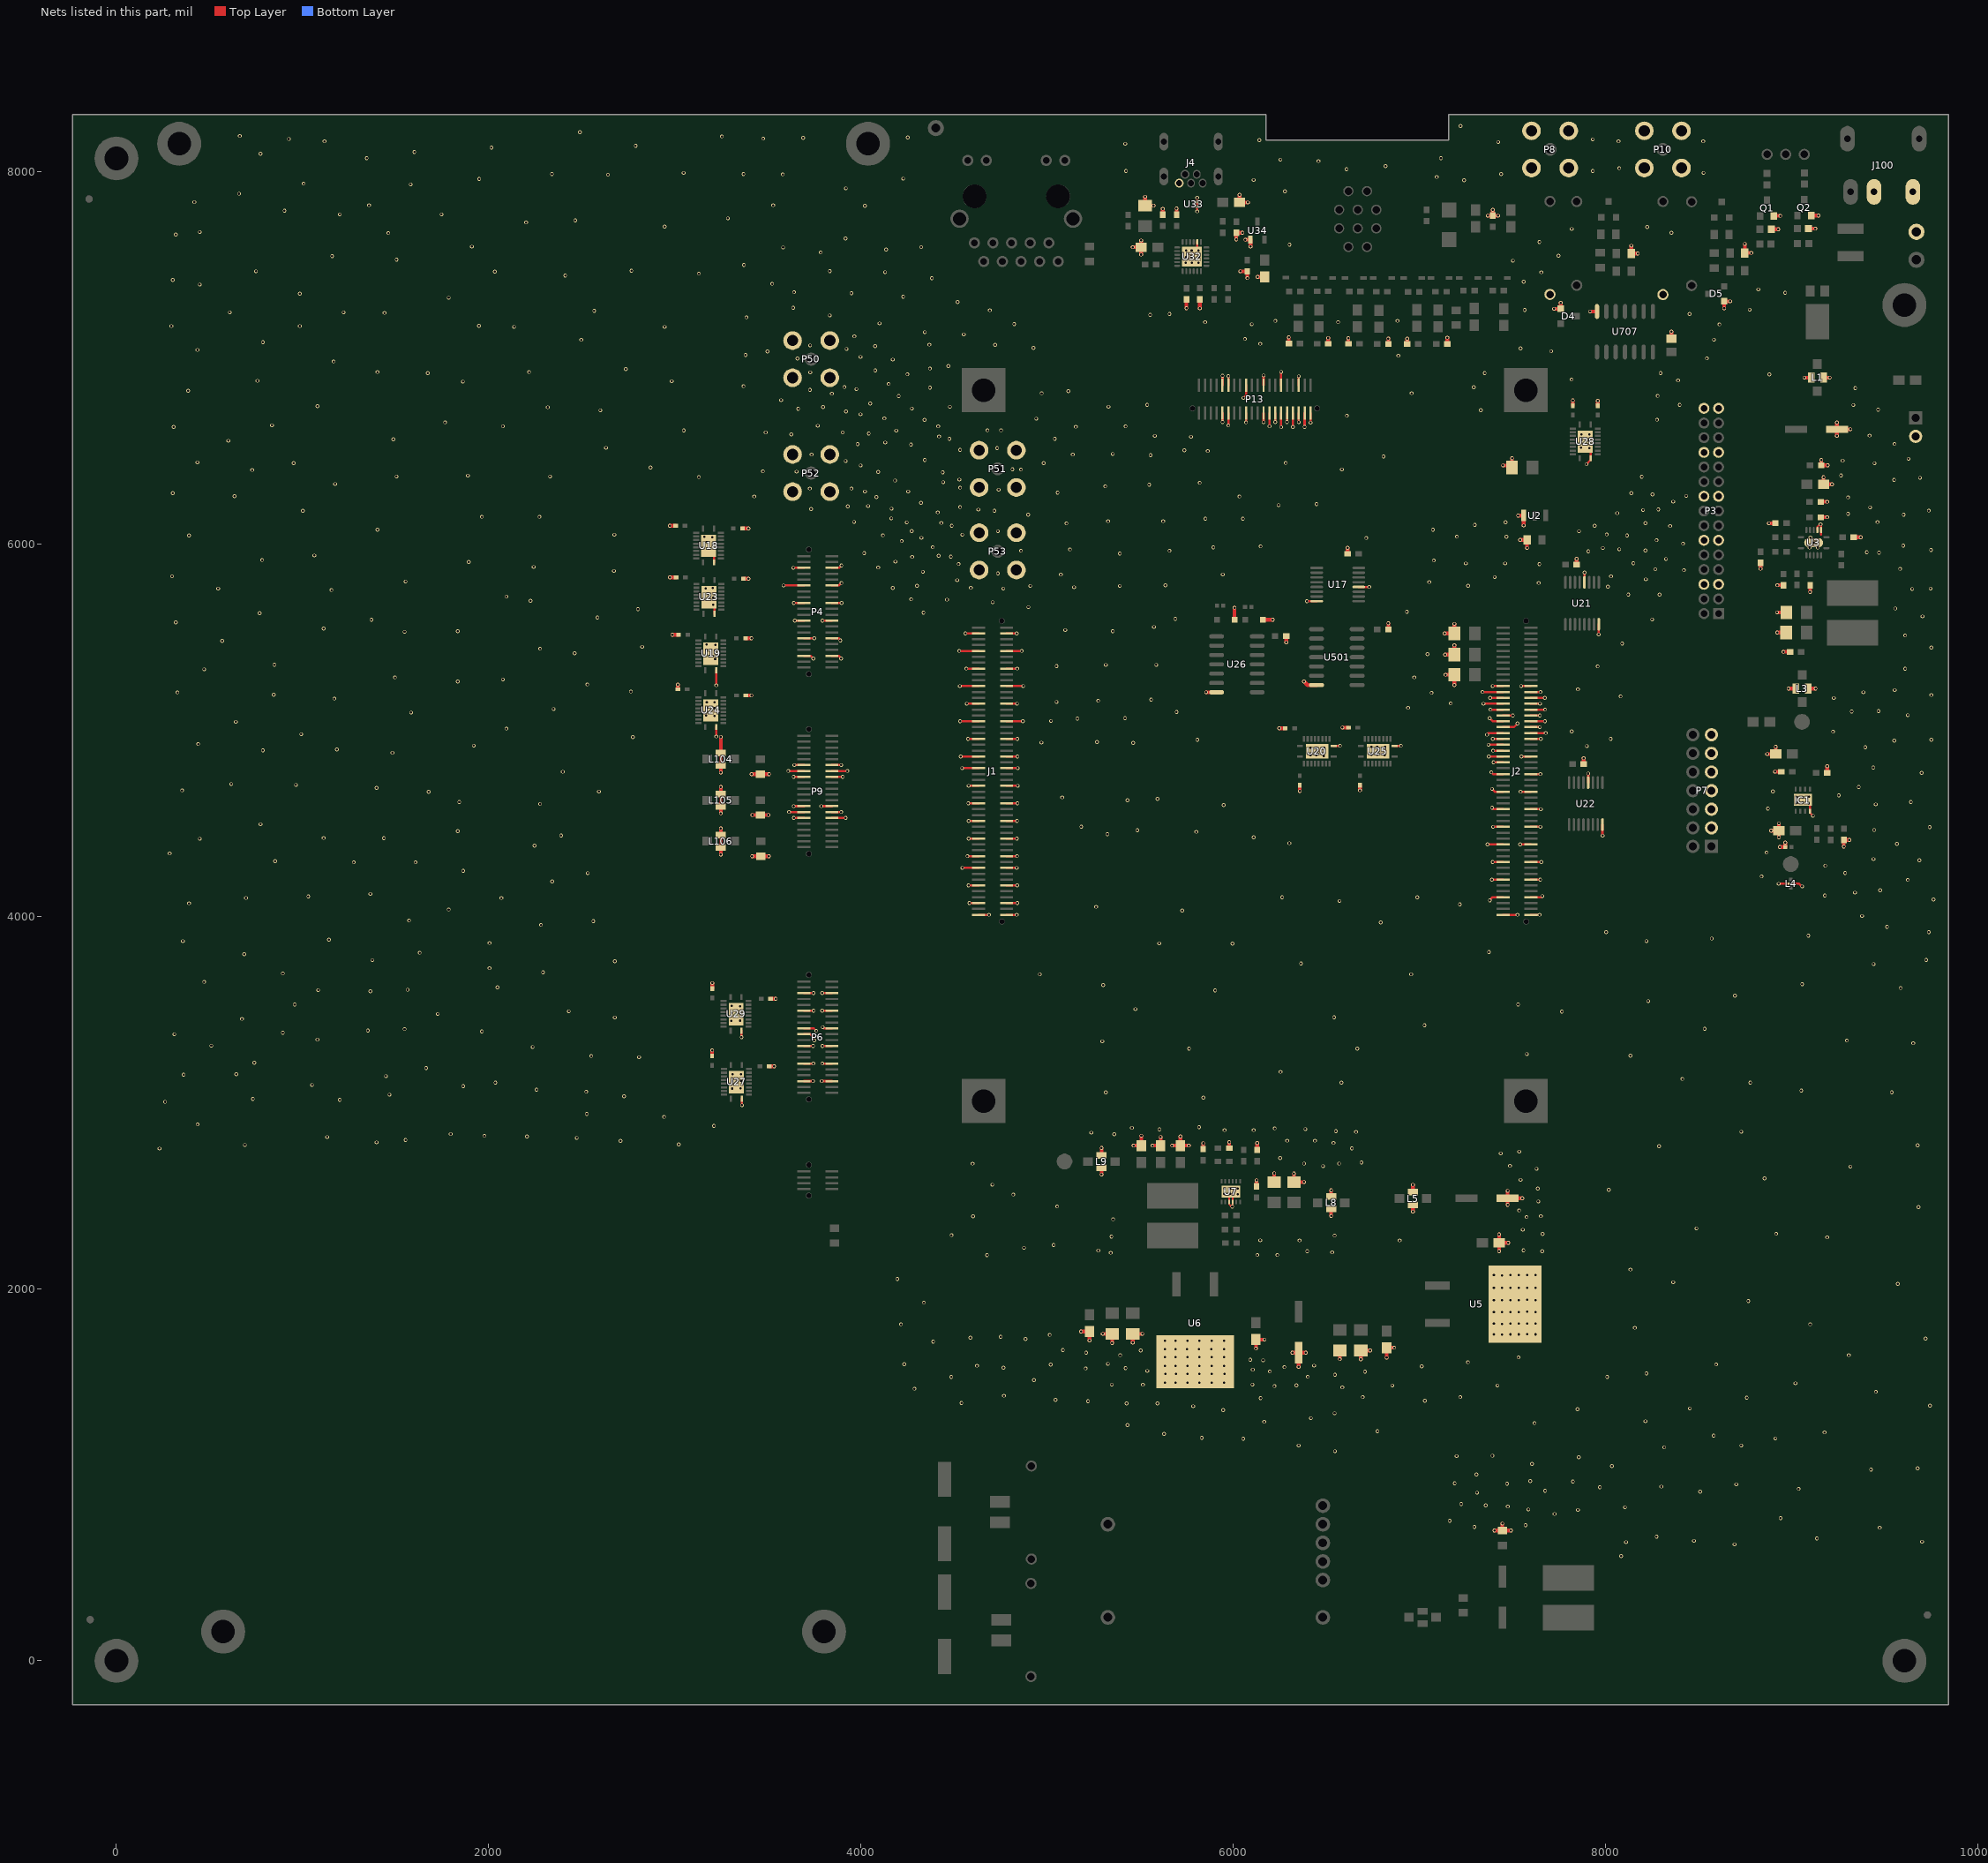
[diagram p0: the nets of this part, all layers, seen from the top]
# Altium PCB MISC82191.PcbDoc (part 5 of 9)
Units mil, origin at the board's own origin, x right, y up, seen from the top; angles counter-clockwise.
Board outline 10078.74 x 8543.31 mil, 4 copper layers (Top Layer, GND, POWER, Bottom Layer); 238 components, 299 nets, 1297 pads, 1665 vias.

## Via types
v1: diameter 20, hole 12, Top Layer to Bottom Layer, 1664 vias
v2: diameter 40, hole 20, Top Layer to Bottom Layer, 1 vias

## Nets (pads, with @x,y where several pads share a name; then routed paths per layer and width w, separated by ;. In a path a pad name is that pad's centre, name@x,y a point inside that pad or via, vN(x,y) a via of type N, cw(c..) or ccw(c..) an arc to the next point about the centre after c; other vN are vias at no path point) (continued)
DGND: C3.2 C4.1 C5.1 C6.1 C7.1 C8.2 C9.2 C10.2 C13.1 C14.1 C15.2 C16.2 C17.2 C18.2 C19.2 C20.2 C21.2 C23.2 C24.1 C25.1 C26.1 C27.1 C35.1 C36.1 C37.1 C38.2 C39.1 C40.1 C41.2 C42.2 C43.2 C47.1 C48.1 C49.1 C50.2 C54.2 C55.2 C59.2 C60.2 C61.1 C66.2 C67.1 C68（NC）.2 C69.1 C70.1 C71.2 C72.1 C73.2 C74.1 C75.2 C76.1 C77.1 C78.2 C79.1 C80.2 C81.1 C82.2 C83.1 C85.2 C86.1 C87.2 C88.1 C89.2 C90.1 C91.2 C95.2 C97.2 C104.1 C105.2 C106.1 C107.1 C108.1 C109.1 C110.1 C111.2 C112.2 C115.2 C116.1 C117.1 C501.1 C502.1 C704.1 C706.1 CN1.2 D2.1 D3.1 D4.1 D5.1 IC1.4 IC1.9 J1.A2 J1.A5 J1.A8 J1.A11 J1.A14 J1.A17 J1.A20 J1.A23 J1.A25 J1.A28 J1.A31 J1.A34 J1.A37 J1.A40 J1.A42 J1.A45 J1.A48 J1.A50 J1.B2 J1.B5 J1.B8 J1.B11 J1.B14 J1.B17 J1.B20 J1.B23 J1.B25 J1.B28 J1.B31 J1.B34 J1.B37 J1.B40 J1.B42 J1.B45 J1.B48 J1.B50 J2.A11 J2.A12 J2.A13 J2.A14 J2.A15 J2.A16 J2.A17 J2.A18 J2.A19 J2.A20 J2.A23 J2.A26 J2.A29 J2.A32 J2.A35 J2.A38 J2.A41 J2.A44 J2.A47 J2.A50 J2.B11 J2.B12 J2.B13 J2.B14 J2.B15 J2.B16 J2.B17 J2.B18 J2.B19 J2.B20 J2.B21 J2.B22 J2.B23 J2.B24 J2.B26 J2.B29 J2.B32 J2.B35 J2.B38 J2.B41 J2.B44 J2.B47 J2.B50 J4.5 J100.2 J100.3 J300.2 L1.2 L1.4 L3.2 L3.4 L4.2 L4.4 L5.2 L5.4 L8.2 L8.4 L9.2 L9.4 L104.2 L104.4 L105.2 L105.4 L106.2 L106.4 P3.5 P3.6 P3.11 P3.12 P3.17 P3.18 P3.23 P3.24 P3.29 P3.30 P4.5 P4.6 P4.11 P4.12 P4.17 P4.18 P4.23 P4.24 P4.29 P4.30 P4.35 P4.36 P6.5 P6.6 P6.11 P6.12 P6.17 P6.18 P6.19 P6.23 P6.24 P6.29 P6.30 P6.35 P6.36 P7.3 P7.5 P7.7 P7.9 P7.11 P7.13 P8.1 P8.2 P8.3 P8.4 P9.11 P9.12 P9.13 P9.14 P9.15 P9.16 P9.25 P9.26 P9.27 P9.28 P9.29 P9.30 P10.1 P10.2 P10.3 P10.4 P13.9 P13.10 P13.11 P13.12 P13.17 P13.18 P13.23 P13.24 P13.25 P13.27 P13.29 P13.30 P13.31 P13.33 P13.35 P13.36 P13.37 P13.39 P50.1 P50.2 P50.3 P50.4 P51.1 P51.2 P51.3 P51.4 P52.1 P52.2 P52.3 P52.4 P53.1 P53.2 P53.3 P53.4 Q1.2 Q2.2 R1.1 R5.2 R7.2 R8.2 R14.2 R27.1 R28.1 R38.1 R42.1 R48.2 RZ1.2 U2.1 U3.2 U3.3 U3.15 U5.4 U6.4 U7.9 U7.10 U7.13 U17.8 U17.12 U18.11 U19.11 U20.11 U21.8 U21.12 U22.8 U22.12 U23.11 U24.11 U25.11 U26.7 U27.11 U28.11 U29.11 U32.2 U32.25 U33.3 U33.4 U34.1 U501.7 U707.7 | length 16609.1
  Top Layer w10: U7.13@5977.54,2490.4 U7.9@5977.54,2465.59 5977.54,2453.4 v1@5989.78,2441.16 ; v1(5994.78,2440.16) 5997.22,2442.6 U7.10@5997.22,2465.59 U7.13@5997.22,2491.72 ; U3.3@9138.55,6074.54 9138.55,6091.93 v1@9152.78,6106.16 ; v1(9155.78,6105.16) 9155.78,6103.16 9158.24,6100.7 U3.2@9158.24,6074.54 9158.24,6048.62
  Top Layer w11: P6.19@3694.21,3366.31 3727.62,3366.31 3748.78,3345.16 v1(3748.78,3334.16) ; P6.17@3694.21,3397.81 3746.13,3397.81 v1(3759.78,3384.16) ; P6.11@3694.21,3492.3 v1(3745.64,3492.3) ; P6.5@3694.21,3586.79 v1(3745.15,3586.79) ; v1(3791.41,3586.79) P6.6@3843.82,3586.79 ; v1(3791.64,3492.3) P6.12@3843.82,3492.3 ; v1(3794.78,3404.16) 3801.13,3397.81 P6.18@3843.82,3397.81 ; IC1.9@9098.55,4592.93 IC1.4@9098.55,4563.16 9098.55,4555.39 v1(9114.78,4539.16)
  Top Layer w12: U18.11@3210.74,5900.68 U18.11@3210.74,5933.11 ; U23.11@3212.83,5624.68 U23.11@3212.83,5657.1 ; v1(3222.78,4965.16) 3222.83,4965.21 U24.11@3222.83,5016.68 ; v1(3222.83,5240.21) U19.11@3222.83,5321.68 ; v1(3358.78,3350.16) 3358.78,3357.16 3358.83,3357.21 U29.11@3358.83,3384.68 ; v1(3360.83,2984.21) U27.11@3360.83,3019.68 ; v1(3584.16,5776.78) P4.11@3694.21,5776.78 ; v1(3609.76,4780.17) P9.13@3694.21,4780.17 ; v1(3614.24,4559.7) P9.27@3694.21,4559.7 ; v1(3636.89,5871.27) P4.5@3694.21,5871.27 ; v1(3638.26,4748.68) P9.15@3694.21,4748.68 ; v1(3638.74,4591.2) P9.25@3694.21,4591.2 ; v1(3638.83,4528.2) P9.29@3694.21,4528.2 ; v1(3638.91,5682.29) P4.17@3694.21,5682.29 ; v1(3642.29,4811.67) P9.11@3694.21,4811.67 ; v1(3644.43,5587.8) P4.23@3694.21,5587.8 ; P6.35@3694.21,3114.35 v1(3742.59,3114.35) ; P6.29@3694.21,3208.83 v1(3744.46,3208.83) ; P6.23@3694.21,3303.32 v1(3742.94,3303.32) ; P4.35@3694.21,5398.83 3729.11,5398.83 v1(3743.78,5384.16) ; P4.29@3694.21,5493.31 v1(3748.62,5493.31) ; v1(3786.74,4591.2) P9.26@3843.82,4591.2 ; v1(3788.97,3114.35) P6.36@3843.82,3114.35 ; v1(3792.1,3208.83) P6.30@3843.82,3208.83 ; v1(3792.94,3303.32) P6.24@3843.82,3303.32 ; v1(3793.43,5587.8) P4.24@3843.82,5587.8 ; P9.30@3843.82,4528.2 v1(3917.83,4528.2) ; P9.28@3843.82,4559.7 v1(3894.32,4559.7) ; P9.16@3843.82,4748.68 v1(3902.26,4748.68) ; P9.14@3843.82,4780.17 v1(3927.76,4780.17) ; P9.12@3843.82,4811.67 v1(3894.29,4811.67) ; P4.36@3843.82,5398.83 3880.11,5398.83 3893.78,5385.16 v1(3893.78,5384.16) ; P4.30@3843.82,5493.31 3879.62,5493.31 3889.78,5483.16 v1(3889.78,5481.16) ; P4.18@3843.82,5682.29 v1(3895.65,5682.29) ; P4.12@3843.82,5776.78 3881.4,5776.78 v1(3894.78,5790.16) ; P4.6@3843.82,5871.27 3881.89,5871.27 v1(3894.78,5884.16) ; v1(4527.94,5425) J1.B5@4632.75,5425 ; v1(4530.92,5236.02) J1.B11@4632.75,5236.02 ; v1(4532.89,5047.05) J1.B17@4632.75,5047.05 ; v1(4535.84,4858.09) J1.B23@4632.75,4858.09 ; v1(4543.72,4795.1) J1.B25@4632.75,4795.1 ; v1(4544.27,4259.67) J1.B42@4632.75,4259.67 ; v1(4561.11,5519.49) J1.B2@4632.75,5519.49 ; v1(4566.13,5330.51) J1.B8@4632.75,5330.51 ; v1(4568.4,5141.53) J1.B14@4632.75,5141.53 ; v1(4572.28,4322.66) J1.B40@4632.75,4322.66 ; v1(4575.18,4952.56) J1.B20@4632.75,4952.56 ; v1(4576.81,4606.13) J1.B31@4632.75,4606.13 ; v1(4577.8,4165.18) J1.B45@4632.75,4165.18 ; v1(4578.24,4700.61) J1.B28@4632.75,4700.61 ; v1(4578.26,4511.64) J1.B34@4632.75,4511.64 ; v1(4578.79,4417.15) J1.B37@4632.75,4417.15 ; v1(4582.31,4070.69) J1.B48@4632.75,4070.69 ; J1.B50@4632.75,4007.7 v1(4687.32,4007.7) ; J1.A50@4782.37,4007.7 v1(4837.32,4007.7) ; J1.A48@4782.37,4070.69 v1(4840.24,4070.69) ; J1.A45@4782.37,4165.18 v1(4839.76,4165.18) ; J1.A42@4782.37,4259.67 v1(4837.29,4259.67) ; J1.A40@4782.37,4322.66 v1(4838.28,4322.66) ; J1.A37@4782.37,4417.15 v1(4837.79,4417.15) ; J1.A34@4782.37,4511.64 v1(4838.3,4511.64) ; J1.A31@4782.37,4606.13 v1(4840.75,4606.13) ; J1.A28@4782.37,4700.61 v1(4842.24,4700.61) ; J1.A25@4782.37,4795.1 v1(4842.72,4795.1) ; J1.A23@4782.37,4858.09 v1(4840.72,4858.09) ; J1.A20@4782.37,4952.56 v1(4840.38,4952.56) ; J1.A17@4782.37,5047.05 v1(4869.89,5047.05) ; J1.A14@4782.37,5141.53 v1(4838.4,5141.53) ; J1.A11@4782.37,5236.02 v1(4871.92,5236.02) ; J1.A8@4782.37,5330.51 v1(4839.13,5330.51) ; J1.A5@4782.37,5425 v1(4863.94,5425) ; J1.A2@4782.37,5519.49 v1(4836.45,5519.49) ; v1(5806.15,7785.79) U33.4@5806.15,7837.57 v1(5806.15,7859.79) ; U32.25@5807.1,7593.48 U32.2@5807.1,7622.16 ; v1(5942.65,6654.03) P13.9@5942.65,6702.82 ; P13.10@5942.65,6852.42 v1(5942.65,6903.03) ; v1(5974.15,6636.53) P13.11@5974.15,6702.82 ; P13.12@5974.15,6852.42 v1(5974.15,6901.53) ; v1(6055.78,6784.16) 6055.78,6786.16 6068.64,6799.02 P13.18@6068.64,6852.42 ; v1(6068.64,6653.02) P13.17@6068.64,6702.82 ; v1(6163.13,6653.81) P13.23@6163.13,6702.82 ; P13.24@6163.13,6852.42 v1(6163.13,6904.81) ; v1(6194.62,6632) P13.25@6194.62,6702.82 ; v1(6226.12,6654.5) P13.27@6226.12,6702.82 ; v1(6257.61,6627.32) P13.29@6257.61,6702.82 ; P13.30@6257.61,6852.42 v1(6257.61,6923.99) ; v1(6288.78,6654.16) 6289.11,6654.49 P13.31@6289.11,6702.82 ; v1(6320.61,6627.98) P13.33@6320.61,6702.82 ; v1(6352.1,6653.48) P13.35@6352.1,6702.82 ; P13.36@6352.1,6852.42 v1(6352.1,6900.48) ; v1(6383.6,6627.98) P13.37@6383.6,6702.82 ; v1(6395.64,5692.02) U17.8@6448.78,5692.02 ; v1(6415.09,6651.47) P13.39@6415.09,6702.82 ; U20.11@6539.91,4915.78 v1(6573.4,4915.78) ; U17.12@6674.43,5768.79 v1(6731.15,5768.79) ; U25.11@6866.91,4915.78 v1(6900.4,4915.78) ; v1(7339.15,5204.53) J2.B12@7449.4,5204.53 ; v1(7344.4,5141.53) J2.B14@7449.4,5141.53 ; v1(7363.78,4975.16) 7372.67,4984.05 J2.B19@7449.4,4984.05 ; v1(7366.28,4385.65) J2.B38@7449.4,4385.65 ; v1(7371.71,4921.09) J2.B21@7449.4,4921.09 ; v1(7372.84,4858.09) J2.B23@7449.4,4858.09 ; v1(7377.78,5064.16) 7394.89,5047.05 J2.B17@7449.4,5047.05 ; v1(7378.78,4085.41) 7378.78,4087.16 7393.81,4102.19 J2.B47@7449.4,4102.19 ; v1(7379.91,5173.03) J2.B13@7449.4,5173.03 ; v1(7381.9,5110.04) J2.B15@7449.4,5110.04 ; v1(7386.78,4773.16) 7396.33,4763.61 J2.B26@7449.4,4763.61 ; v1(7390.26,4196.68) J2.B44@7449.4,4196.68 ; v1(7390.78,4583.16) 7399.31,4574.63 J2.B32@7449.4,4574.63 ; v1(7390.78,4684.16) 7405.82,4669.12 J2.B29@7449.4,4669.12 ; v1(7393.79,4291.16) J2.B41@7449.4,4291.16 ; v1(7393.92,5236.02) J2.B11@7449.4,5236.02 ; v1(7394.18,4952.56) J2.B20@7449.4,4952.56 ; v1(7395.8,4480.14) J2.B35@7449.4,4480.14 ; v1(7396.21,4889.59) J2.B22@7449.4,4889.59 ; v1(7398.22,4826.6) J2.B24@7449.4,4826.6 ; J2.B50@7449.4,4007.7 v1(7527.32,4007.7) ; J2.B18@7449.4,5015.55 7508.17,5015.55 v1(7527.78,5035.16) ; J2.B16@7449.4,5078.54 v1(7502.4,5078.54) ; v1(7541.28,4385.65) J2.A38@7599.01,4385.65 ; v1(7543.82,4669.12) J2.A29@7599.01,4669.12 ; v1(7546.92,5236.02) J2.A11@7599.01,5236.02 ; v1(7548.84,4858.09) J2.A23@7599.01,4858.09 ; J2.A50@7599.01,4007.7 v1(7646.24,4007.7) ; J2.A47@7599.01,4102.19 7654.81,4102.19 v1(7660.78,4108.16) ; J2.A44@7599.01,4196.68 v1(7649.51,4196.68) ; J2.A41@7599.01,4291.16 v1(7654.77,4291.16) ; J2.A35@7599.01,4480.14 v1(7650.76,4480.14) ; J2.A32@7599.01,4574.63 v1(7653.31,4574.63) ; J2.A26@7599.01,4763.61 v1(7650.23,4763.61) ; J2.A20@7599.01,4952.56 v1(7653.38,4952.56) ; J2.A19@7599.01,4984.05 v1(7678.67,4984.05) ; J2.A18@7599.01,5015.55 v1(7647.39,5015.55) ; J2.A17@7599.01,5047.05 7674.67,5047.05 v1(7674.78,5047.16) ; J2.A16@7599.01,5078.54 v1(7647.4,5078.54) ; J2.A15@7599.01,5110.04 v1(7675.66,5110.04) ; J2.A14@7599.01,5141.53 v1(7648.4,5141.53) ; J2.A13@7599.01,5173.03 v1(7673.91,5173.03) ; J2.A12@7599.01,5204.53 v1(7651.41,5204.53) ; U21.12@7887.15,5793.81 v1(7887.15,5846.53) ; v1(7897.78,6428.16) 7920.83,6451.21 U28.11@7920.83,6460.06 U28.11@7920.83,6495.1 ; v1(8930.14,4174.52) L4.2@8983.97,4174.52 ; L4.4@9007.58,4174.52 9040.42,4174.52 9054.78,4160.16 v1(9056.78,4160.16)
  Top Layer w13: v1(7963.92,5513.3) U21.8@7963.92,5568.16
  Top Layer w14: U22.12@7907.15,4717.81 v1(7907.15,4766.53) ; U22.8@7983.92,4492.16 7983.92,4432.41 v1(7984.78,4432.41)
  Top Layer w20: v1(2972.78,6097.16) C72.1@3004.78,6097.16 ; v1(2973.78,5820.16) C79.1@3006.78,5820.16 ; v1(2986.78,5512.16) C74.1@3019.78,5512.16 ; C81.1@3016.78,5219.16 v1(3016.78,5244.16) ; C86.1@3200.78,3249.16 v1(3200.78,3280.16) ; C90.1@3201.78,3611.16 v1(3201.78,3641.16) ; v1(3246.95,4330.58) L106.4@3246.95,4369.32 v1(3246.95,4472.24) ; v1(3246.95,4552.58) L105.4@3246.95,4589.32 v1(3246.95,4695.24) ; v1(3246.95,4771.58) L104.4@3246.95,4810.32 v1(3246.95,4963.24) ; C71.2@3363.78,6083.16 v1(3395.78,6083.16) ; C78.2@3368.78,5813.16 v1(3395.78,5813.16) ; C73.2@3380.78,5493.16 v1(3411.78,5493.16) ; C80.2@3381.78,5186.16 v1(3411.78,5186.16) ; v1(3412.41,4762.78) C704.1@3458.78,4762.78 v1(3506.15,4762.78) ; v1(3415.41,4321.78) C97.2@3462.78,4321.78 v1(3505.41,4321.78) ; v1(3416.41,4543.78) C706.1@3459.78,4543.78 v1(3503.15,4543.78) ; C85.2@3507.78,3194.16 v1(3533.78,3194.16) ; C89.2@3514.78,3556.16 v1(3541.78,3556.16) ; v1(5182.45,1768.83) C37.1@5227.59,1768.83 v1(5227.59,1720.97) ; v1(5292.76,2612.18) L9.4@5292.76,2648.37 ; L9.2@5292.76,2715.29 v1(5292.76,2755.14) ; v1(5299.45,1756.83) C36.1@5349.59,1756.83 v1(5349.59,1707.35) ; v1(5460.59,1709.35) C35.1@5460.59,1756.83 v1(5511.45,1756.83) ; v1(5460.78,7594.16) C105.2@5505.78,7594.16 ; v1(5464.11,2767.83) C48.1@5506.59,2767.83 v1(5506.59,2820.97) ; v1(5505.78,7554.16) C105.2@5505.78,7594.16 ; v1(5505.78,7630.16) C105.2@5505.78,7594.16 ; v1(5526.78,7865.16) C111.2@5526.78,7817.16 v1(5572.78,7817.16) ; v1(5566.11,2767.83) C47.1@5610.59,2767.83 v1(5610.59,2813.97) ; C112.2@5621.78,7768.16 v1(5621.78,7800.16) ; v1(5672.11,2767.83) C49.1@5716.59,2767.83 ; C106.1@5695.78,7768.16 v1(5695.78,7802.16) ; v1(5716.59,2817.35) C49.1@5716.59,2767.83 ; v1(5748.78,7266.16) R48.2@5748.78,7313.16 ; v1(5761.45,2767.83) C49.1@5716.59,2767.83 ; v1(5820.78,7265.16) C107.1@5820.78,7314.16 ; C50.2@5838.78,2749.16 v1(5838.78,2780.16) ; v1(5854.78,5203.16) U26.7@5910.78,5203.16 ; R14.2@5978.59,2753.83 v1(5978.59,2785.97) ; D2.1@6007.22,5592.16 v1(6007.22,5657.6) ; v1(6016.78,7636.16) C109.1@6016.78,7671.16 v1(6049.78,7671.16) ; v1(6033.78,7875.16) C104.1@6033.78,7834.16 v1(6078.78,7834.16) ; v1(6037.78,7464.16) 6055.78,7464.16 C108.1@6075.78,7464.16 v1(6075.78,7428.16) ; v1(6065.78,7634.16) U34.1@6092.78,7634.16 v1(6092.78,7597.16) ; v1(6122.59,1677.35) C39.1@6122.59,1725.83 v1(6168.11,1725.83) ; C41.2@6125.59,2548.83 v1(6125.59,2581.35) ; C40.1@6128.59,2744.83 v1(6128.59,2781.35) ; v1(6130.78,7434.16) C110.1@6168.78,7434.16 ; D3.1@6159.22,5592.16 v1(6212.78,5592.16) ; C43.2@6220.59,2571.83 v1(6220.59,2618.97) ; v1(6247.78,5009.16) C75.2@6279.78,5009.16 ; v1(6284.78,5471.16) C77.1@6284.78,5504.16 ; C54.2@6298.78,7076.16 v1(6298.78,7110.16) ; v1(6317.47,1655.47) C38.2@6351.36,1655.47 ; v1(6326.59,2617.97) C42.2@6326.59,2571.83 v1(6381.11,2571.83) ; v1(6351.36,1578.57) C38.2@6351.36,1655.47 ; v1(6357.78,4672.16) C76.1@6357.78,4704.16 ; v1(6379.78,5261.16) 6399.21,5241.72 U501.7@6447.66,5241.72 ; v1(6390.09,1655.47) C38.2@6351.36,1655.47 ; C55.2@6510.78,7075.16 v1(6510.78,7106.16) ; v1(6526.42,2390.52) L8.2@6526.42,2427.37 ; L8.4@6526.42,2494.29 v1(6526.42,2527.52) ; v1(6572.59,1620.97) C27.1@6572.59,1667.45 ; v1(6586.78,5013.16) C82.2@6618.78,5013.16 ; C61.1@6614.78,5947.16 v1(6614.78,5979.16) ; C59.2@6618.78,7075.16 v1(6618.78,7105.16) ; v1(6680.78,4676.16) C83.1@6680.78,4704.16 ; v1(6685.59,1619.97) C26.1@6685.59,1667.45 v1(6735.11,1667.45) ; v1(6824.4,1628.61) C25.1@6824.4,1682.09 v1(6864.92,1682.09) ; C501.1@6833.78,5541.16 v1(6833.78,5574.16) ; C60.2@6833.78,7074.16 v1(6833.78,7103.16) ; C66.2@6934.78,7074.16 v1(6934.78,7102.16) ; v1(6965.8,2413.42) L5.2@6965.8,2450.27 ; L5.4@6965.8,2517.19 v1(6965.8,2557.38) ; v1(7135.8,5519.18) C115.2@7188.21,5519.18 v1(7188.21,5570.59) ; v1(7138.76,5405.18) C116.1@7188.21,5405.18 v1(7188.21,5455.72) ; v1(7140.76,5297.18) C117.1@7188.21,5297.18 v1(7188.21,5241.59) ; C68（NC）.2@7150.78,7074.16 v1(7150.78,7108.16) ; v1(7367.78,7763.16) C67.1@7394.78,7763.16 ; v1(7394.78,7795.16) C67.1@7394.78,7763.16 ; v1(7403.15,699.78) RZ1.2@7445.78,699.78 ; v1(7422.78,7763.16) C67.1@7394.78,7763.16 ; v1(7428.73,2200.11) C24.1@7428.73,2245.59 ; v1(7428.73,2290.45) C24.1@7428.73,2245.59 ; v1(7445.78,737.41) RZ1.2@7445.78,699.78 ; v1(7449.78,6421.16) 7486.78,6421.16 C3.2@7497.78,6410.16 v1(7497.78,6460.16) ; v1(7474.09,2449.09) C23.2@7474.09,2485.36 ; v1(7474.09,2524.47) C23.2@7474.09,2485.36 ; v1(7478.59,2245.59) C24.1@7428.73,2245.59 ; v1(7492.41,699.78) RZ1.2@7445.78,699.78 ; v1(7530.89,6152.27) U2.1@7560.47,6152.27 v1(7560.47,6098.85) ; v1(7541.78,6021.16) C4.1@7578.78,6021.16 v1(7578.78,5978.16) ; v1(7553.82,2485.36) C23.2@7474.09,2485.36 ; v1(7723.78,7263.16) D4.1@7759.78,7263.16 v1(7759.78,7295.16) ; C88.1@7824.78,6742.16 v1(7824.78,6771.16) ; C69.1@7844.78,5888.16 v1(7844.78,5920.16) ; C70.1@7882.78,4818.16 v1(7882.78,4849.16) ; v1(7917.15,7248.78) U707.7@7954.78,7248.78 ; C87.2@7958.78,6742.16 v1(7958.78,6768.16) ; v1(8138.78,7602.16) C91.2@8138.78,7560.16 v1(8173.78,7560.16) ; C502.1@8354.78,7102.78 v1(8354.78,7140.41) ; v1(8637.78,7265.16) D5.1@8637.78,7303.16 v1(8669.78,7303.16) ; v1(8748.78,7611.16) C95.2@8748.78,7563.16 v1(8783.78,7563.16) ; v1(8833.03,5866.41) C21.2@8833.03,5898.41 ; v1(8868.78,4871.16) C5.1@8914.78,4871.16 v1(8914.78,4910.16) ; v1(8877.78,6111.16) R7.2@8912.78,6111.16 ; v1(8889.78,4459.16) C14.1@8931.78,4459.16 ; R28.1@8890.33,7690.36 v1(8929.23,7690.36) ; Q1.2@8905.33,7762.36 v1(8939.23,7762.36) ; v1(8910.78,4776.16) C6.1@8944.78,4776.16 ; v1(8921.78,5632.16) C18.2@8971.78,5632.16 ; v1(8922.78,5524.16) C19.2@8970.78,5524.16 ; v1(8923.78,5778.16) C20.2@8956.78,5778.16 ; v1(8931.78,4424.16) C14.1@8931.78,4459.16 ; v1(8931.78,4499.16) C14.1@8931.78,4459.16 ; v1(8936.78,4372.16) C13.1@8965.74,4372.16 v1(8965.74,4395.12) ; v1(8955.78,5420.16) C17.2@8991.78,5420.16 ; v1(8983.61,5223.33) L3.2@9023.32,5223.33 ; v1(9068.68,6893.26) L1.2@9105.06,6893.26 ; L3.4@9090.24,5223.33 v1(9128.61,5223.33) ; R27.1@9091.33,7693.36 v1(9127.83,7693.36) ; v1(9099.78,5742.16) R5.2@9099.78,5778.16 ; Q2.2@9106.33,7763.36 v1(9144.73,7763.36) ; C9.2@9156.78,6143.16 v1(9190.78,6143.16) ; C10.2@9156.78,6226.16 v1(9191.78,6226.16) ; v1(9159.52,6450.9) C16.2@9159.52,6422.09 v1(9194.71,6422.09) ; v1(9171.52,6358.42) C8.2@9171.52,6320.09 v1(9216.85,6320.09) ; L1.4@9171.98,6893.26 v1(9204.88,6893.26) ; C7.1@9191.78,4770.16 v1(9191.78,4805.16) ; v1(9243.88,6580.06) C15.2@9243.88,6615.86 ; v1(9243.88,6652.26) C15.2@9243.88,6615.86 ; v1(9280.78,4374.16) R1.1@9280.78,4410.16 v1(9310.78,4410.16) ; v1(9316.08,6615.86) C15.2@9243.88,6615.86 ; R8.2@9333.78,6036.16 v1(9371.78,6036.16)
  Bottom Layer w12: v1@3221.78,4966.16 v1(3222.78,4965.16)